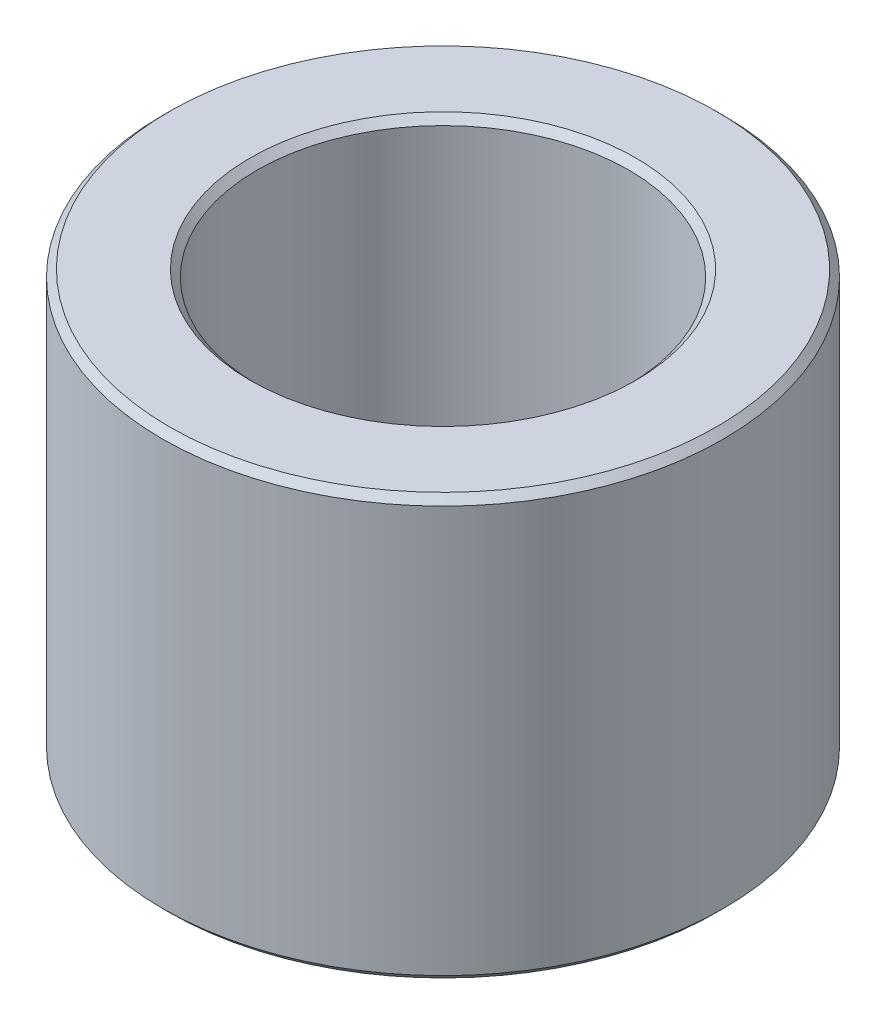
SolidWorks part; units mm, degrees
material "S45C"
ref_plane "Front Plane" through (0, 0, 0) normal (0, 0, 1) x (1, 0, 0)
ref_plane "Top Plane" through (0, 0, 0) normal (0, 1, 0) x (1, 0, 0)
ref_plane "Right Plane" through (0, 0, 0) normal (1, 0, 0) x (0, 0, -1)
sketch "Sketch1" plane through (0, 0, 0) normal (0, 1, 0) x (1, 0, 0)
  circle A0 centre (0, 0) radius 8
  circle A1 centre (0, 0) radius 5.3
  dimension "D1" = 16
  dimension "D2" = 10.6
extrude "Boss-Extrude1" add sketch "Sketch1" along normal blind 12
chamfer "Chamfer1" distance 0.2 angle 45 4 edges at (0, 0, 5.3) (0, 0, 8) (0, 12, 8) (0, 12, 5.3)
